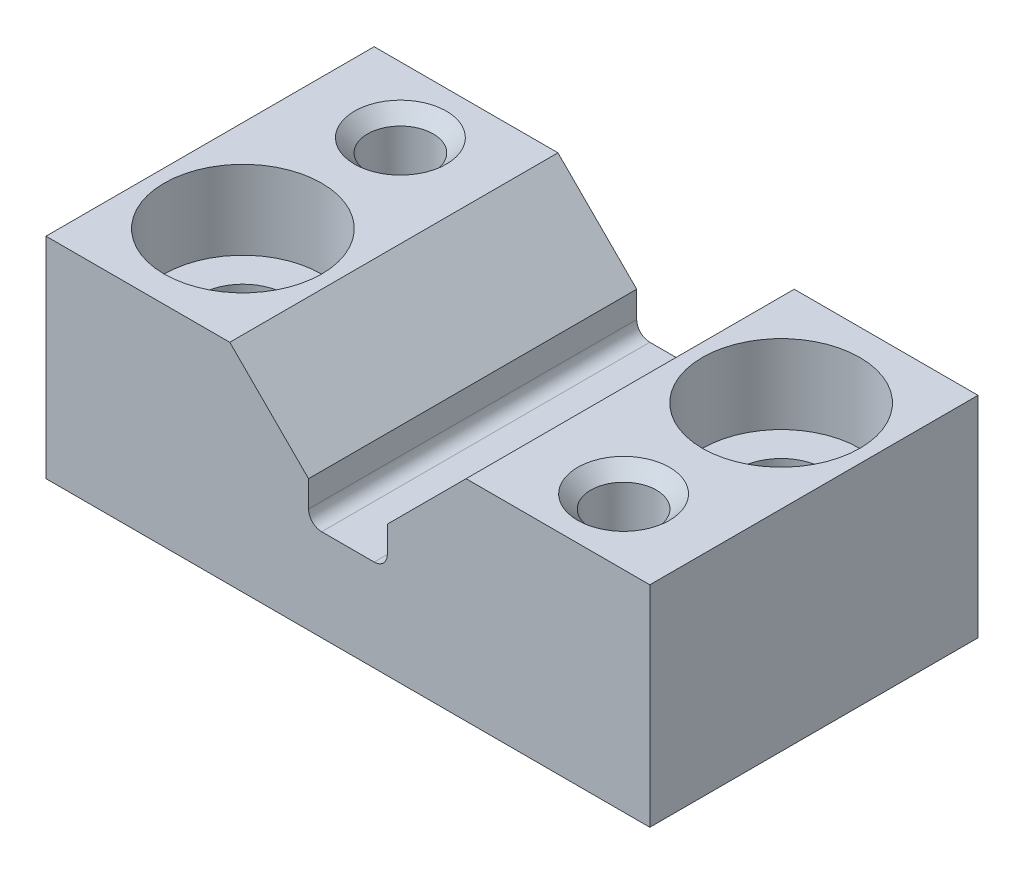
SolidWorks part; units mm, degrees
extrude "Boss-Extrude" add sketch "Sketch1" along normal blind 25
sketch "Sketch1" plane through (0, 0, 0) normal (0, 0, 1) x (1, 0, 0)
  line L1 (-23, 0) -> (23, 0)
  line L2 (-23, 0) -> (-23, -16)
  line L3 (-23, -16) -> (23, -16)
  line L4 (23, 0) -> (23, -16)
extrude "Cut-Extrude1" cut sketch "Sketch2" against normal through all
sketch "Sketch2" plane through (0, 0, 25) normal (0, 0, 1) x (1, 0, 0)
  line L0 (0, 30) -> (0, -70) construction
  line L1 (-3, -9) -> (3, -9)
  line L2 (-9, 0) -> (9, 0)
  line L3 (23, 0) -> (-23, 0) construction
  line L4 (9, 0) -> (3, -6)
  line L5 (3, -6) -> (3, -9)
  line L6 (-9, 0) -> (-3, -6)
  line L7 (-3, -6) -> (-3, -9)
  point P9 (0, -9)
extrude "Cut-Extrude4" cut sketch "Sketch4" against normal through all
sketch "Sketch4" plane through (0, 0, 0) normal (0, 1, 0) x (-1, 0, 0)
  line L0 (9, 0) -> (23, 0) construction
  line L1 (-16, 70) -> (-16, -17.4052) construction
  line L2 (40, 17) -> (80, 17) construction
  line L4 (40, 5) -> (80, 5) construction
  line L5 (0, -20) -> (0, 70) construction
  line L6 (16, 70) -> (16, -17.4052) construction
  line L7 (-20, 20) -> (-76.4032, 20) construction
  line L8 (-20, 8) -> (-76.4032, 8) construction
  line L9 (9, 25) -> (23, 25) construction
  circle A0 centre (16, 17) radius 3.3
  circle A1 centre (16, 5) radius 2.5
  circle A2 centre (-16, 20) radius 2.5
  circle A3 centre (-16, 8) radius 3.3
  point P0 (16, 0)
material "S45C"
ref_plane "Front" through (0, 0, 0) normal (0, 0, 1) x (1, 0, 0)
ref_plane "Top" through (0, 0, 0) normal (0, 1, 0) x (1, 0, 0)
ref_plane "Right" through (0, 0, 0) normal (1, 0, 0) x (0, 0, -1)
fillet "Fillet1" radius 1 1 edges at (-3, -9, 12.5)
fillet "Fillet2" radius 1 1 edges at (3, -9, 12.5)
sketch "Sketch5" plane through (0, 0, 0) normal (0, 1, 0) x (-1, 0, 0)
  line L0 (0, 70) -> (0, -20) construction
  line L1 (-16, 65.5158) -> (-16, -20) construction
  line L2 (16, 72.6533) -> (16, -20) construction
  circle A0 centre (16, 17) radius 6
  circle A1 centre (-16, 8) radius 6
  circle A2 centre (-16, 8) radius 3.3 construction
  circle A3 centre (16, 17) radius 3.3 construction
extrude "Cut-Extrude5" cut sketch "Sketch5" against normal blind 6
chamfer "Chamfer1" distance 1 angle 45 1 edges at (16, 0, 22.5)
chamfer "Chamfer2" distance 1 angle 45 1 edges at (-16, 0, 7.5)
chamfer "Chamfer3" distance 1 angle 45 1 edges at (16, -16, 22.5)
chamfer "Chamfer4" distance 1 angle 45 1 edges at (-16, -16, 7.5)
equation "\"D1@Sketch1\" = \"L@Sketch1\" / 2"
equation "\"D2@Sketch2\" = \"N@Sketch2\" / 2"
equation "\"D1@Sketch2\" = \"b@Sketch2\" / 2"
equation "\"D4@Sketch2\" = \"D3@Sketch2\""
equation "\"D4@Sketch4\" = \"d@Sketch4\""
equation "\"D3@Sketch4\" =\"d1@Sketch4\""
equation "\"D5@Sketch4\" = \"A2@Sketch4\""
equation "\"D1@Sketch5\" = \"d2@Sketch5\""
equation "\"D1@Fillet2\" = \"r@Fillet1\""
equation "\"D3@Sketch2\" = \"h1@Sketch2\" - \"N@Sketch2\"  / 2 + \"b@Sketch2\" / 2"
